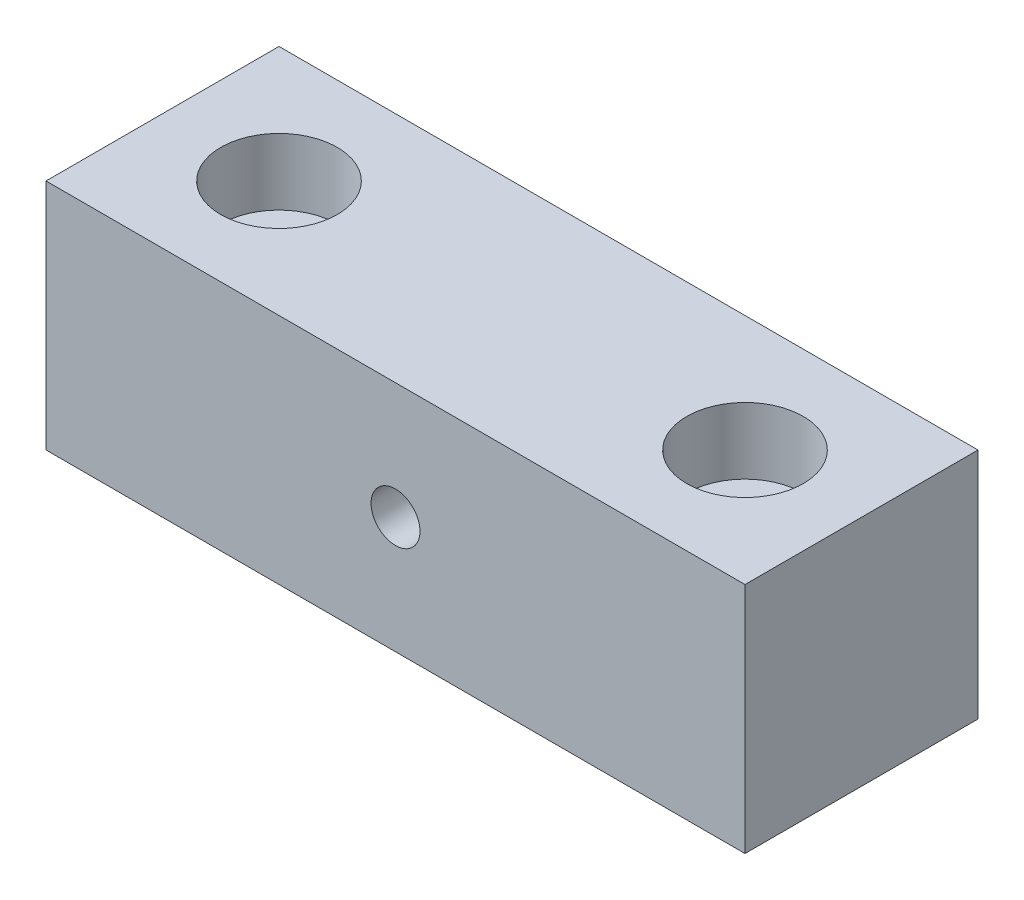
from build123d import *

# Parameters (mm, degrees)
SKETCH_1_W                = 60
SKETCH_1_H                = 20
EXTRUDE_1_DEPTH           = 10
HOLE_WIZARD_1_D           = 5.5
HOLE_WIZARD_1_CBORE_D     = 10
HOLE_WIZARD_1_CBORE_DEPTH = 5.7
HOLE_WIZARD_M5_1_D        = 4.2


with BuildPart() as part:
    # 草图1 → 凸台-拉伸1 (new, symmetric)
    with BuildSketch(Plane(origin=(0, 0, 0), x_dir=(1, 0, 0), z_dir=(0, 1, 0))):
        Rectangle(SKETCH_1_W, SKETCH_1_H)
    extrude(amount=EXTRUDE_1_DEPTH, both=True)

    # 打孔尺寸(%根据)内六角圆柱头螺钉的类型1 (through all)
    with Locations(Plane(origin=(0, 10, 0), x_dir=(1, 0, 0), z_dir=(0, 1, 0))):
        with Locations((20, 0), (-20, 0)):
            CounterBoreHole(HOLE_WIZARD_1_D / 2, HOLE_WIZARD_1_CBORE_D / 2, HOLE_WIZARD_1_CBORE_DEPTH)

    # M5 螺纹孔1 (through all)
    with Locations(Plane.XY.offset(10)):
        with Locations((0, 0)):
            Hole(HOLE_WIZARD_M5_1_D / 2)


solid = part.part
